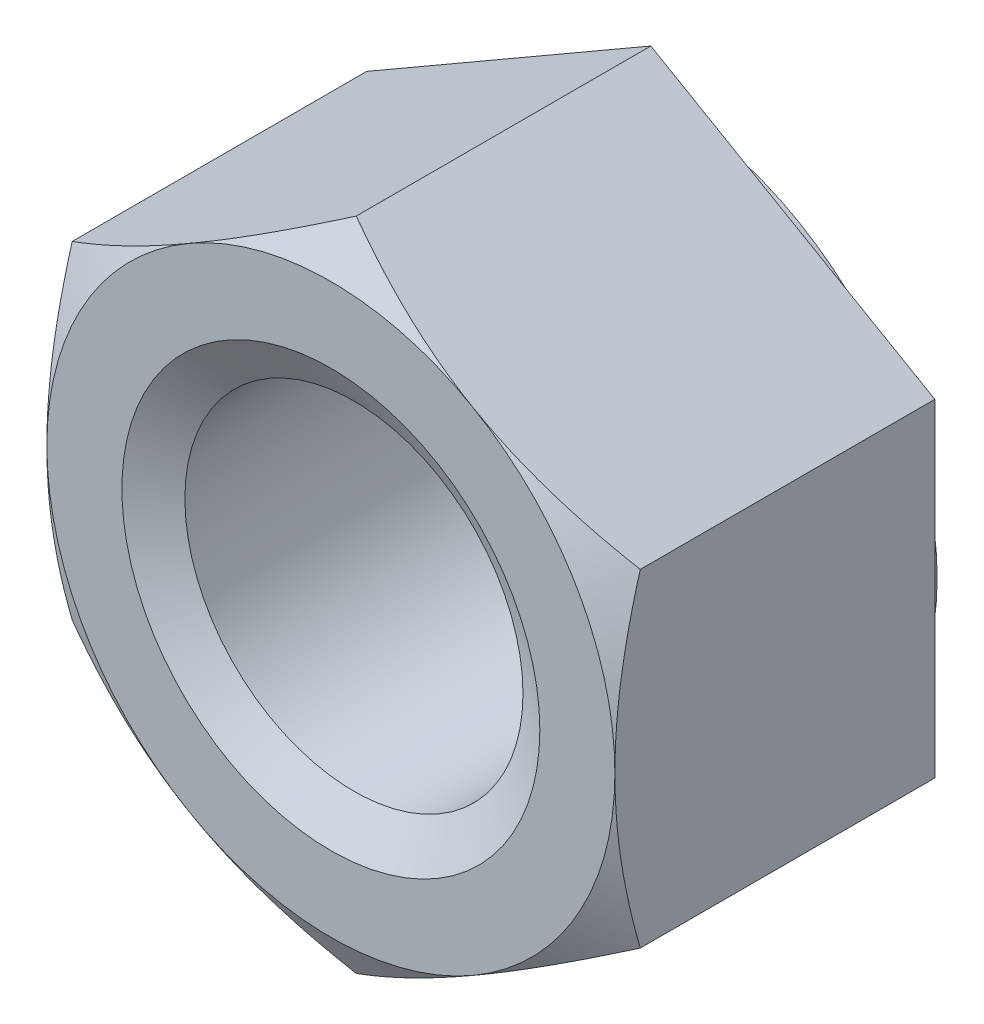
from build123d import *

# Parameters (mm, degrees)
SKETCH_3_R          = 13.105625
EXTRUDE_1_DEPTH     = 25.6
SKETCH_5_R          = 38.1375
SKETCH_5_R_2        = 22.018695891
CUT_EXTRUDE_1_DEPTH = 5.12
CUT_EXTRUDE_1_DRAFT = -60
SKETCH_6_W          = 0.8
SKETCH_6_H          = 4.025


with BuildPart() as part:
    # 草图3 → 凸台-拉伸1 (new body)
    with BuildSketch(Plane.XY):
        Polygon((0, 25.425), (-22.018695891, 12.7125), (-22.018695891, -12.7125), (0, -25.425), (22.018695891, -12.7125), (22.018695891, 12.7125), align=None)
        Circle(SKETCH_3_R, mode=Mode.SUBTRACT)
    extrude(amount=-EXTRUDE_1_DEPTH)

    # 草图4 → 切除-旋转1 (revolve, cut)
    with BuildSketch(Plane(origin=(0, 0, 0), x_dir=(0, 0, -1), z_dir=(1, 0, 0)), mode=Mode.PRIVATE) as cut_revolve_1_sk:
        Polygon((0, 16.2), (1.786538239, 13.105625), (1.786538239, 0), (0, 0), align=None)
        Polygon((25.6, 0), (25.6, 16.2), (23.813461761, 13.105625), (23.813461761, 0), align=None)
    revolve(cut_revolve_1_sk.sketch.rotate(Axis((0, 0, 0), (0, 0, -1)), 90), axis=Axis((0, 0, 0), (0, 0, -1)), mode=Mode.SUBTRACT)


with BuildPart() as cut_extrude_1_tool:
    # 草图5 → 切除-拉伸1 (with draft: the straight prism first)
    with BuildSketch(Plane.XY):
        Circle(SKETCH_5_R)
        Circle(SKETCH_5_R_2, mode=Mode.SUBTRACT)
    extrude(amount=-CUT_EXTRUDE_1_DEPTH)
    # 切除-拉伸1: the draft: its side faces are tilted about the plane it starts from
    cut_extrude_1_sides = [cut_extrude_1_tool.faces().sort_by_distance(p)[0] for p in [
        (-38.1375, 0, -2.56),
        (-22.018695891, 0, -2.56),
    ]]
    draft(cut_extrude_1_sides, Plane.XY, CUT_EXTRUDE_1_DRAFT)


with BuildPart() as part_1:
    add(part.part)

    # 切除-拉伸1: cut by cut_extrude_1_tool
    add(cut_extrude_1_tool.part, mode=Mode.SUBTRACT)

    # 草图6 → 切除-旋转2 (revolve, cut)
    with BuildSketch(Plane(origin=(0, 0, 0), x_dir=(0, 0, -1), z_dir=(1, 0, 0)), mode=Mode.PRIVATE) as cut_revolve_2_sk:
        with Locations((25.2, 23.4125)):
            Rectangle(SKETCH_6_W, SKETCH_6_H)
    revolve(cut_revolve_2_sk.sketch.rotate(Axis((0, 0, 0), (0, 0, -1)), 90), axis=Axis((0, 0, 0), (0, 0, -1)), mode=Mode.SUBTRACT)


solid = part_1.part
